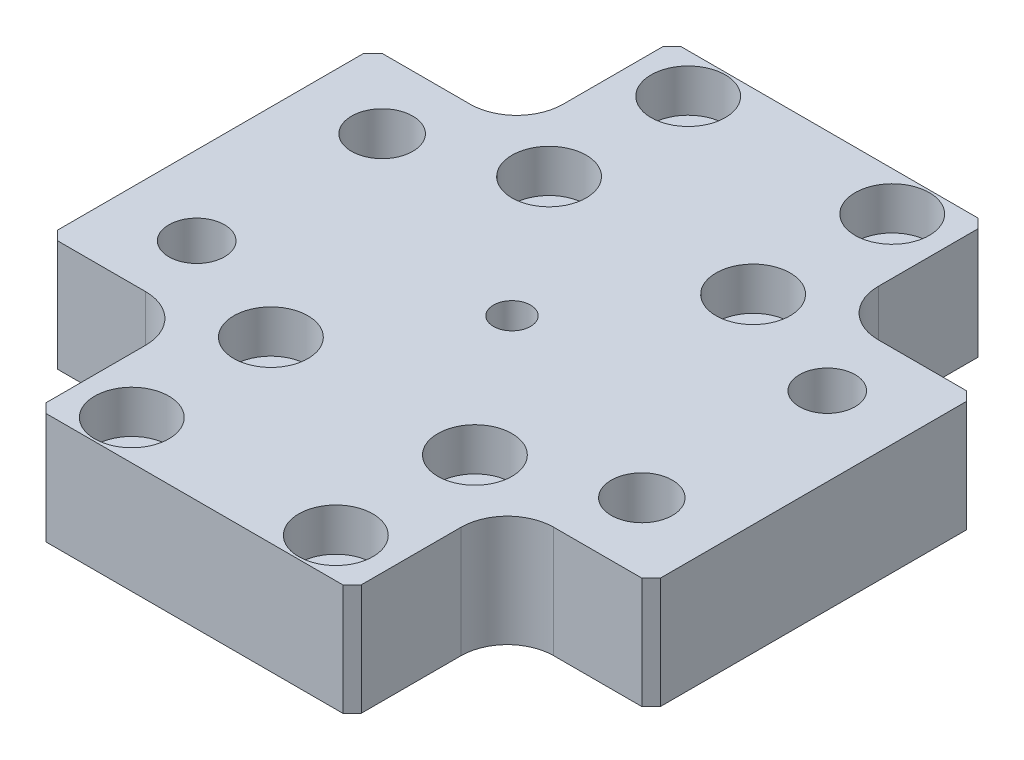
SolidWorks part; units mm, degrees
material "A6061"
ref_plane "前基準面" through (0, 0, 0) normal (0, 0, 1) x (1, 0, 0)
ref_plane "上基準面" through (0, 0, 0) normal (0, 1, 0) x (1, 0, 0)
ref_plane "右基準面" through (0, 0, 0) normal (1, 0, 0) x (0, 0, -1)
sketch "草图1" plane through (0, 0, 0) normal (0, 1, 0) x (1, 0, 0)
  line L1 (-32.5, -34.25) -> (32.5, -34.25)
  line L2 (-32.5, -34.25) -> (-32.5, 34.25)
  line L3 (-32.5, 34.25) -> (32.5, 34.25)
  line L4 (32.5, -34.25) -> (32.5, 34.25)
  line L5 (-32.5, -34.25) -> (32.5, 34.25) construction
  line L6 (-32.5, 34.25) -> (32.5, -34.25) construction
  circle A0 centre (0, 0) radius 2
  point P0 (0, 0)
  dimension "D3" = 4
  dimension "D1" = 65
  dimension "D2" = 68.5
extrude "凸台-拉伸1" add sketch "草图1" along normal mid plane 12
sketch "草图2" plane through (0, -6, 0) normal (0, 1, 0) x (1, 0, 0)
  line L0 (0, 39.8262) -> (0, 0) construction
  line L1 (0, 0) -> (-41.7993, 0) construction
  line L3 (24, -10) -> (-24, -10) construction
  line L4 (24, -10) -> (24, 10) construction
  line L5 (24, 10) -> (-24, 10) construction
  line L6 (-24, -10) -> (-24, 10) construction
  point P0 (-24, 10)
  point P19 (24, -10)
  dimension "D1" = 20
  dimension "D2" = 48
hole_wizard "M6 六角圆柱头螺钉的柱形沉头孔1" positions "草图2" profile "草图3" counterbore size "M6" standard "GB" end condition through all
sketch "草图3" plane through (-24, -6, -10) normal (1, 0, 0) x (0, 0, -1)
  line L0 (0, 0) -> (0, 12)
  line L1 (0, 12) -> (3.3, 12)
  line L3 (3.3, 12) -> (3.3, 6.8)
  line L4 (3.3, 6.8) -> (5.5, 6.8)
  line L5 (5.5, 6.8) -> (5.5, 0)
  line L7 (5.5, 0) -> (0, 0)
  line L11 (0, -6.35) -> (0, 107.95) construction
  dimension "通孔孔直径" = 6.6
  dimension "通孔孔深度" = 12
  dimension "柱形沉头孔直径" = 11
  dimension "柱形沉头孔深度" = 6.8
sketch "草图4" plane through (0, 6, 0) normal (0, 1, 0) x (1, 0, 0)
  line L0 (0, 25.9571) -> (0, -22.5) construction
  line L1 (0, -22.5) -> (-37.0517, -22.5) construction
  line L2 (0, 0) -> (-38.8438, 0) construction
  point P0 (-11, -15)
  point P10 (-11, -30)
  point P11 (11, -30)
  point P12 (11, -15)
  point P21 (11, 15)
  point P22 (11, 30)
  point P23 (-11, 30)
  point P24 (-11, 15)
  dimension "D1" = 22
  dimension "D2" = 15
  dimension "D3" = 45
hole_wizard "M4 六角圆柱头螺钉的柱形沉头孔1" positions "草图4" profile "草图5" counterbore size "M4" standard "GB" end condition through all
sketch "草图5" plane through (-11, 6, 15) normal (1, 0, 0) x (0, 0, 1)
  line L0 (0, 0) -> (0, 12)
  line L1 (0, 12) -> (2.25, 12)
  line L3 (2.25, 12) -> (2.25, 4.6)
  line L4 (2.25, 4.6) -> (4, 4.6)
  line L5 (4, 4.6) -> (4, 0)
  line L7 (4, 0) -> (0, 0)
  line L11 (0, -6.35) -> (0, 107.95) construction
  dimension "通孔孔直径" = 4.5
  dimension "通孔孔深度" = 12
  dimension "柱形沉头孔直径" = 8
  dimension "柱形沉头孔深度" = 4.6
sketch "草图6" plane through (0, 6, 0) normal (0, 1, 0) x (1, 0, 0)
  line L0 (32.5, 34.25) -> (-32.5, 34.25) construction
  line L1 (-32.5, 34.25) -> (-17, 34.25)
  line L2 (-32.5, 34.25) -> (-32.5, 17.5)
  line L3 (-32.5, 17.5) -> (-22, 17.5)
  line L4 (-17, 34.25) -> (-17, 22.5)
  line L5 (-32.5, 34.25) -> (-32.5, -34.25) construction
  line L6 (0, 56.6769) -> (0, 0) construction
  line L7 (0, 0) -> (-35.7167, 0) construction
  line L8 (-17, -34.25) -> (-17, -22.5)
  line L9 (-32.5, -17.5) -> (-22, -17.5)
  line L10 (-32.5, -34.25) -> (-32.5, -17.5)
  line L11 (-32.5, -34.25) -> (-17, -34.25)
  line L12 (32.5, -34.25) -> (17, -34.25)
  line L13 (32.5, -34.25) -> (32.5, -17.5)
  line L14 (32.5, -17.5) -> (22, -17.5)
  line L15 (17, -34.25) -> (17, -22.5)
  line L16 (17, 34.25) -> (17, 22.5)
  line L17 (32.5, 17.5) -> (22, 17.5)
  line L18 (32.5, 34.25) -> (32.5, 17.5)
  line L19 (32.5, 34.25) -> (17, 34.25)
  arc A0 (-22, 17.5) -> (-17, 22.5) centre (-22, 22.5) ccw
  arc A1 (-22, -17.5) -> (-17, -22.5) centre (-22, -22.5) cw
  arc A2 (22, -17.5) -> (17, -22.5) centre (22, -22.5) ccw
  arc A3 (22, 17.5) -> (17, 22.5) centre (22, 22.5) cw
  dimension "D1" = 5
  dimension "D2" = 34
  dimension "D3" = 35
extrude "切除-拉伸1" cut sketch "草图6" against normal through all both and the other way through all
hole_wizard "Ø6.0mm 暗销孔1" positions "草图7" profile "草图8" hole size "Ø6.0" standard "GB" end condition up to next
sketch "草图7" plane through (0, -6, 0) normal (0, -1, 0) x (-1, 0, 0)
  line L0 (24, 10) -> (24, -10) construction
  line L1 (24, -10) -> (-24, -10) construction
  line L2 (-24, -10) -> (-24, 10) construction
  line L3 (-24, 10) -> (24, 10) construction
  point P0 (-24, 10)
  point P5 (24, -10)
  point P19 (24, -10)
sketch "草图8" plane through (24, -6, -10) normal (1, 0, 0) x (0, 0, -1)
  line L0 (0, 0) -> (0, 12)
  line L1 (0, 12) -> (3, 12)
  line L2 (3, 12) -> (3, 0)
  line L5 (3, 0) -> (0, 0)
  line L11 (0, -6.35) -> (0, 107.95) construction
  dimension "通孔孔直径" = 6
  dimension "通孔孔深度" = 12
chamfer "倒角1" distance 1 angle 45 9 edges at (17, 0, 34.25) (32.5, 0, 17.5) (32.5, 0, -17.5) (17, 0, -34.25) (-17, 0, -34.25) (-32.5, 0, -17.5) (-32.5, 0, 17.5) (-17, 0, 34.25) (0, -6, 2)
sketch "草图9" plane through (0, -6, 0) normal (0, -1, 0) x (1, 0, 0)
  circle A0 centre (0, 0) radius 7.5
  dimension "D1" = 15
extrude "切除-拉伸2" cut sketch "草图9" against normal blind 2
